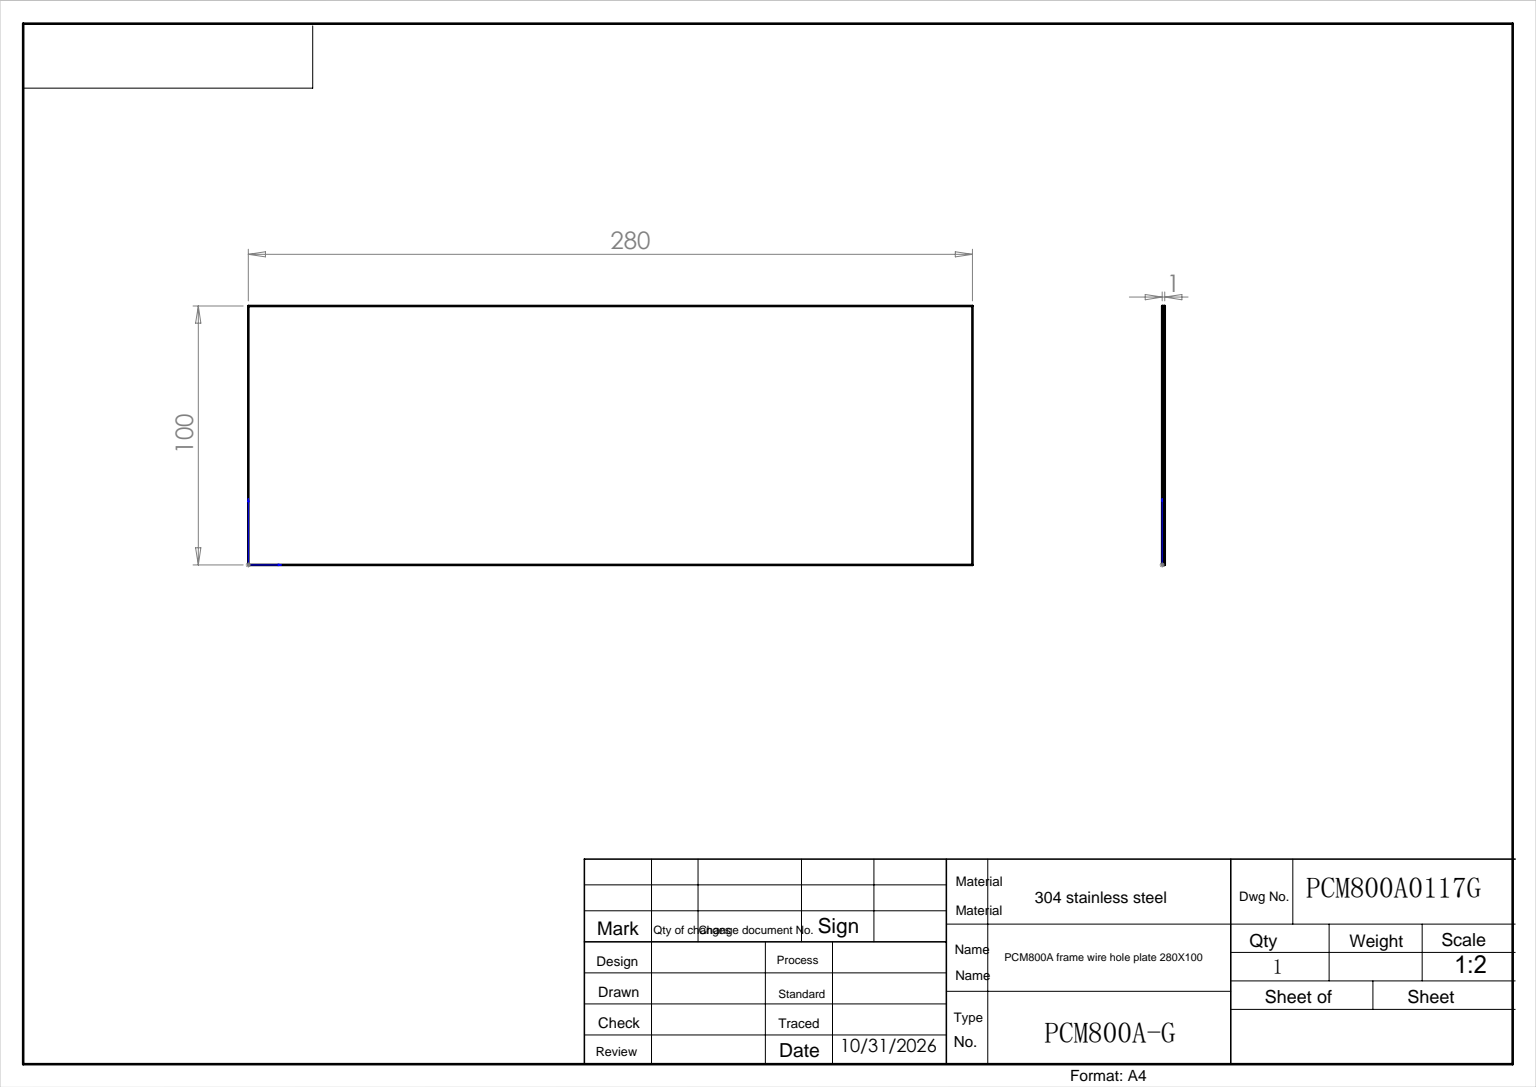
SolidWorks part; units mm, degrees
ref_plane "前视基准面" through (0, 0, 0) normal (0, 0, 1) x (1, 0, 0)
ref_plane "上视基准面" through (0, 0, 0) normal (0, 1, 0) x (1, 0, 0)
ref_plane "右视基准面" through (0, 0, 0) normal (1, 0, 0) x (0, 0, -1)
sketch "草图1" plane through (0, 0, 0) normal (0, 0, 1) x (1, 0, 0)
  line L0 (140, 100) -> (140, 22.8403) construction
  line L1 (0, 0) -> (280, 0)
  line L2 (0, 0) -> (0, 100)
  line L3 (0, 100) -> (280, 100)
  line L4 (280, 0) -> (280, 100)
  line L5 (0, 50) -> (114.8394, 50) construction
  line L6 (0, 0) -> (280, 100) construction
  dimension "D1" = 280
  dimension "D2" = 100
extrude "凸台-拉伸1" add sketch "草图1" along normal blind 1
